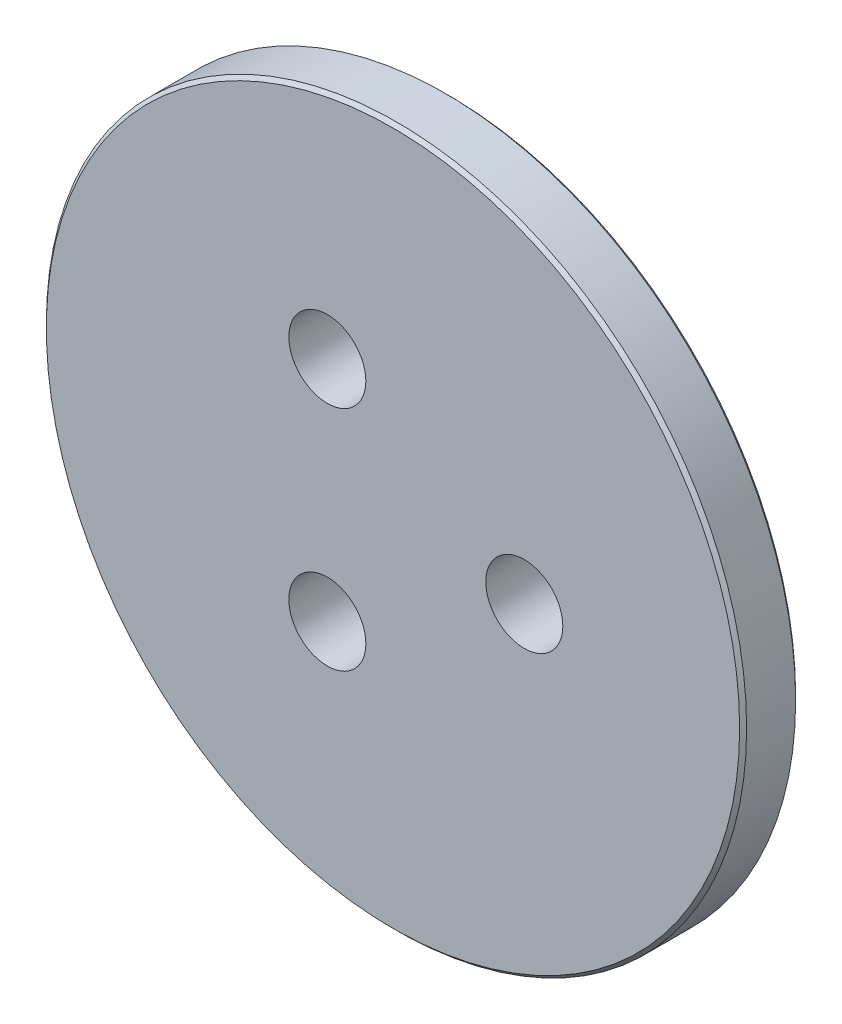
from build123d import *

# Parameters (mm, degrees)
SKETCH1_R           = 100
BOSS_EXTRUDE1_DEPTH = 16
SKETCH2_R           = 11
CUT_EXTRUDE1_DEPTH  = 143.323574997
CIRPATTERN1_COUNT   = 3
CHAMFER1_SIZE       = 1


with BuildPart() as part:
    # Sketch1 → Boss-Extrude1 (new body)
    with BuildSketch(Plane.XY):
        Circle(SKETCH1_R)
    extrude(amount=BOSS_EXTRUDE1_DEPTH)

    # Sketch2 → Cut-Extrude1 (cut, through all)
    with BuildSketch(Plane.XY.offset(16)):
        with Locations((37.5, 0)):
            Circle(SKETCH2_R)
    cut_extrude1 = extrude(amount=-CUT_EXTRUDE1_DEPTH, mode=Mode.SUBTRACT)

    # CirPattern1: Cut-Extrude1 ×3 about axis
    cirpattern1_axis = Axis((0, 0, 0), (0, 0, 1))
    for i in range(1, CIRPATTERN1_COUNT):
        add(cut_extrude1.rotate(cirpattern1_axis, i * 360 / CIRPATTERN1_COUNT), mode=Mode.SUBTRACT)

    # Chamfer1
    chamfer1_edges = [part.edges().sort_by_distance(p)[0] for p in [
        (-100, 0, 0),
        (-100, 0, 16),
    ]]
    chamfer(chamfer1_edges, length=CHAMFER1_SIZE)


solid = part.part
